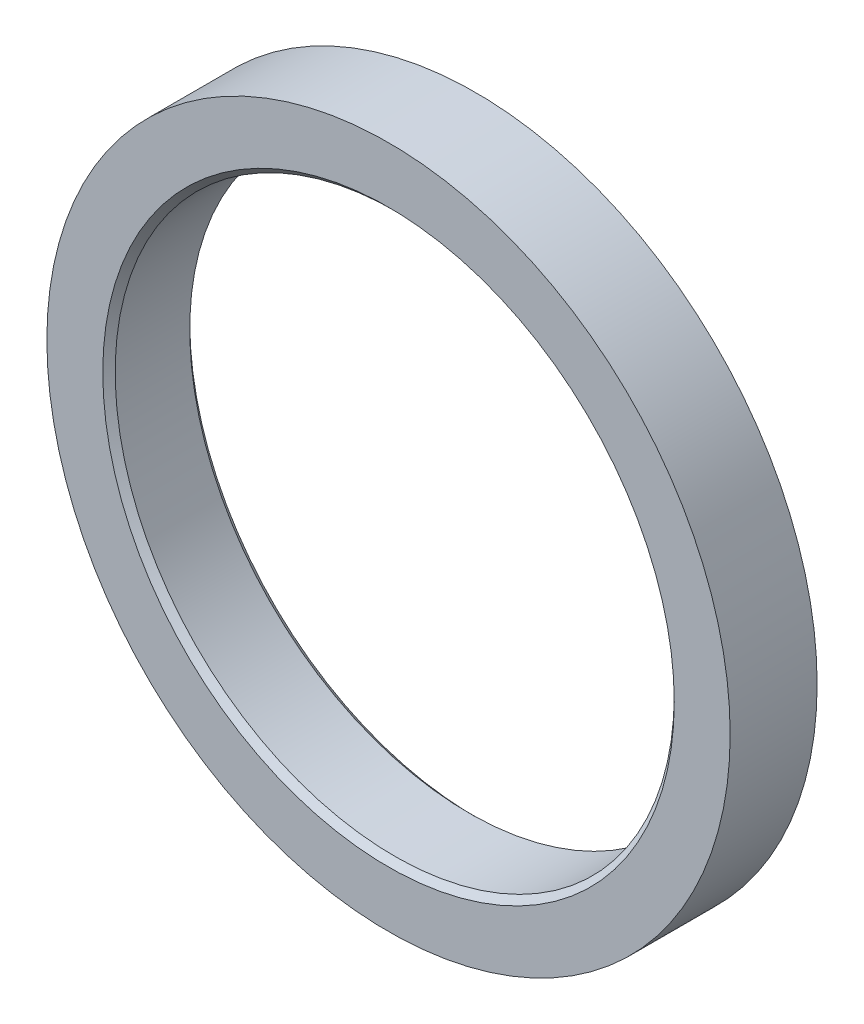
from build123d import *


with BuildPart() as part:
    # Sketch1 → Revolve1 (revolve)
    with BuildSketch(Plane(origin=(0, 22.743963655, 0), x_dir=(1, 0, 0), z_dir=(0, 1, 0))):
        Polygon((598.730642584, 329.192981355), (599.230642584, 328.692981355), (603.730642584, 328.692981355), (603.730642584, 335.692981355), (599.230642584, 335.692981355), (598.730642584, 335.192981355), align=None)
    revolve(axis=Axis((576.230642584, 22.743963655, -335.692981355), (0, 0, 1)))


solid = part.part
